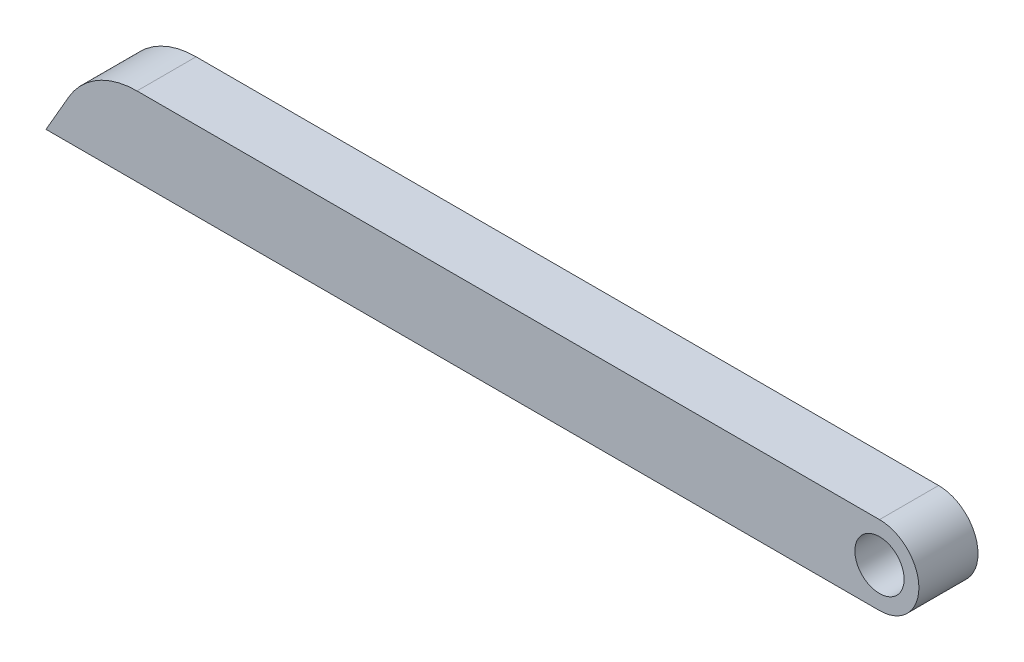
from build123d import *

# Parameters (mm, degrees)
SKETCH1_R           = 0.625
BOSS_EXTRUDE2_DEPTH = 1.5
SKETCH3_R           = 0.75
SKETCH3_R_2         = 0.4
CUT_EXTRUDE1_DEPTH  = 0.5
FILLET1_R           = 2


with BuildPart() as part:
    # Sketch1 → Boss-Extrude2 (new body)
    with BuildSketch(Plane.XY):
        with BuildLine():
            Line((0, 0), (20, 0))
            ThreePointArc((20, 0), (21, -1), (20, -2))
            Line((20, -2), (-1.154700538, -2))
            Line((-1.154700538, -2), (0, 0))
        make_face()
        with Locations((20, -1)):
            Circle(SKETCH1_R, mode=Mode.SUBTRACT)
    extrude(amount=BOSS_EXTRUDE2_DEPTH)

    # Sketch3 → Cut-Extrude1 (cut, symmetric)
    # profile 1 of 5: a face of its own
    with BuildSketch(Plane(origin=(0, 0, 0.75), x_dir=(-1, 0, 0), z_dir=(0, 0, -1))):
        with BuildLine():
            ThreePointArc((-1.371206885, -0.874999993), (-1.096687833, -0.600480945), (-0.721687836, -0.5))
            Line((-0.721687836, -0.5), (-1.154700538, -0.5))
            Line((-1.154700538, -0.5), (-1.371206885, -0.874999993))
        make_face()
    # profile 2 of 5: a face of its own
    with BuildSketch(Plane(origin=(0, 0, 0.75), x_dir=(-1, 0, 0), z_dir=(0, 0, -1))):
        with BuildLine():
            ThreePointArc((-0.721687836, -0.5), (-0.346687831, -0.60048095), (-0.072168777, -0.875000011))
            Line((-0.072168777, -0.875000011), (-0.288675135, -0.5))
            Line((-0.288675135, -0.5), (-0.721687836, -0.5))
        make_face()
    # profile 3 of 5: a face of its own
    with BuildSketch(Plane(origin=(0, 0, 0.75), x_dir=(-1, 0, 0), z_dir=(0, 0, -1))):
        with BuildLine():
            Line((-0.721687836, -2), (0.577350269, -2))
            Line((0.577350269, -2), (-0.072168777, -0.875000011))
            ThreePointArc((-0.072168777, -0.875000011), (0.002756535, -1.055885722), (0.028312164, -1.25))
            ThreePointArc((0.028312164, -1.25), (-0.191357751, -1.780330086), (-0.721687836, -2))
        make_face()
    # profile 4 of 5: a face of its own
    with BuildSketch(Plane(origin=(0, 0, 0.75), x_dir=(-1, 0, 0), z_dir=(0, 0, -1))):
        with BuildLine():
            Line((-2.020725942, -2), (-0.721687836, -2))
            ThreePointArc((-0.721687836, -2), (-1.371206891, -1.624999997), (-1.371206885, -0.874999993))
            Line((-1.371206885, -0.874999993), (-2.020725942, -2))
        make_face()
    # profile 5 of 5: a face of its own
    with BuildSketch(Plane(origin=(0, 0, 0.75), x_dir=(-1, 0, 0), z_dir=(0, 0, -1))):
        with Locations((-0.721687836, -1.25)):
            Circle(SKETCH3_R)
        with Locations((-0.721687836, -1.25)):
            Circle(SKETCH3_R_2, mode=Mode.SUBTRACT)
    extrude(amount=CUT_EXTRUDE1_DEPTH, both=True, mode=Mode.SUBTRACT)

    # Fillet1
    fillet1_edges = [part.edges().sort_by_distance(p)[0] for p in [
        (0, 0, 0.75),
    ]]
    fillet(fillet1_edges, radius=FILLET1_R)


solid = part.part
